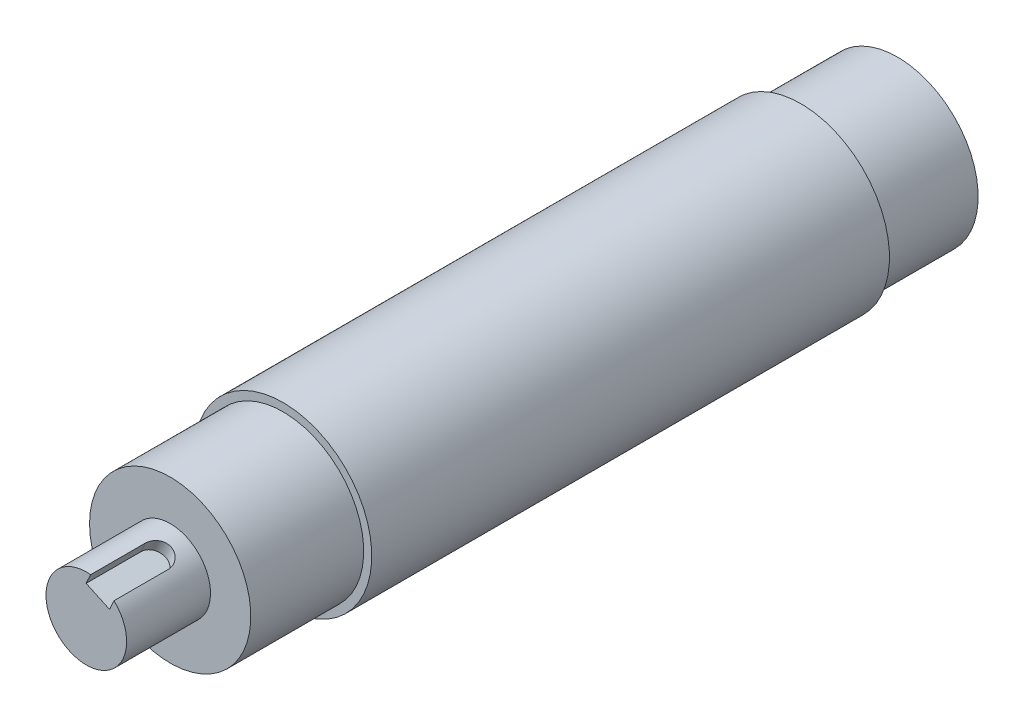
from build123d import *

# Parameters (mm, degrees)
CUT_EXTRUDE_2_DEPTH = 6
CUT_EXTRUDE_3_DEPTH = 7.3


with BuildPart() as part:
    # 草图1 → 旋转1 (revolve)
    with BuildSketch(Plane(origin=(0, 0, 0), x_dir=(1, 0, 0), z_dir=(0, 1, 0))):
        Polygon((-25, 34), (-25, 4), (-27.5, 4), (-27.5, -156.5), (-25, -156.5), (-25, -191.5), (-12.5, -191.5), (-12.5, -217.5), (0, -217.5), (0, 34), align=None)
    revolve(axis=Axis((0, 0, 0), (0, 0, 1)))

    # 草图3 → 切除-拉伸2 (cut)
    with BuildSketch(Plane(origin=(0, -27.5, 0), x_dir=(-1, 0, 0), z_dir=(0, -1, 0))):
        with BuildLine():
            Line((8, -66.5), (8, -112.5))
            ThreePointArc((8, -112.5), (0, -120.5), (-8, -112.5))
            Line((-8, -112.5), (-8, -66.5))
            ThreePointArc((-8, -66.5), (0, -58.5), (8, -66.5))
        make_face()
    extrude(amount=-CUT_EXTRUDE_2_DEPTH, mode=Mode.SUBTRACT)

    # 草图4 → 切除-拉伸3 (cut)
    with BuildSketch(Plane(origin=(6.627052614, 14.343018289, 0), x_dir=(0.9077859676868876, -0.41943370974539124, 0), z_dir=(-0.4194337097453913, -0.9077859676868877, 0))):
        with BuildLine():
            Line((4, 219.353468604), (4, 200.5))
            ThreePointArc((4, 200.5), (0, 196.5), (-4, 200.5))
            Line((-4, 200.5), (-4, 219.353468604))
            ThreePointArc((-4, 219.353468604), (0, 223.353468604), (4, 219.353468604))
        make_face()
    extrude(amount=CUT_EXTRUDE_3_DEPTH, mode=Mode.SUBTRACT)


solid = part.part
